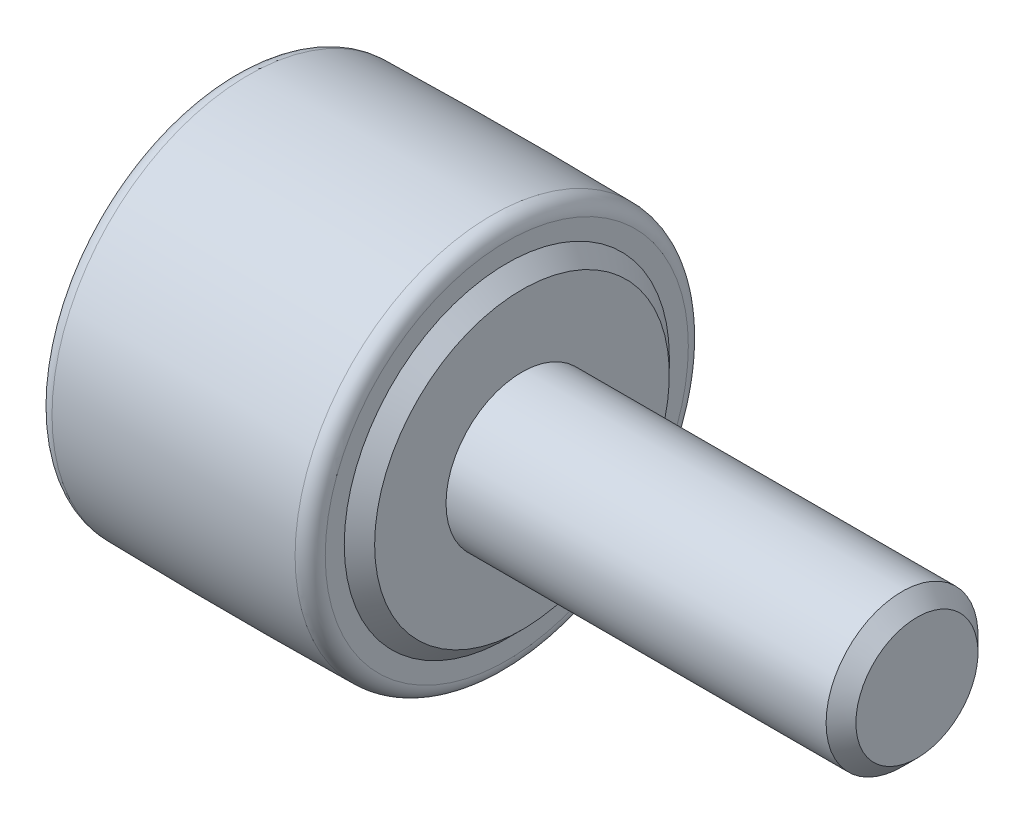
SolidWorks part; units mm, degrees
material "S45C"
ref_plane "Front Plane" through (0, 0, 0) normal (0, 0, 1) x (1, 0, 0)
ref_plane "Top Plane" through (0, 0, 0) normal (0, 1, 0) x (1, 0, 0)
ref_plane "Right Plane" through (0, 0, 0) normal (1, 0, 0) x (0, 0, -1)
ref_plane "Plane1" through (0, 0, 0) normal (0, 0, 1) x (1, 0, 0)
sketch "Sketch1" plane through (0, 0, 0) normal (0, 0, 1) x (1, 0, 0)
  line L0 (-10, 0) -> (-10, 4.85)
  line L1 (-10, 4.85) -> (-9.5, 5.35)
  line L2 (-9.5, 5.35) -> (-9.5, 5.9594)
  line L3 (-0.5, 5.9754) -> (-0.5, 5.35)
  line L4 (-0.5, 5.35) -> (0, 4.85)
  line L5 (0, 4.85) -> (0, 2.5)
  line L6 (0, 2.5) -> (12.5095, 2.5)
  line L7 (12.5095, 2.5) -> (13, 2.0095)
  line L8 (13, 2.0095) -> (13, 0)
  line L9 (13, 0) -> (-10, 0)
  line L10 (13, 0) -> (-10, 0) construction
  arc A0 (-9.5, 5.9594) -> (-9.009, 6.4593) centre (-9, 5.9594) cw
  arc A1 (-9.009, 6.4593) -> (-0.993, 6.4754) centre (-4.5, -243.5) cw
  arc A2 (-0.993, 6.4754) -> (-0.5, 5.9754) centre (-1, 5.9754) cw
revolve "Revolve1" add sketch "Sketch1" angle 360 about L10
ref_plane "Plane2" through (-10, 0, 0) normal (-1, 0, 0) x (0, 0, 1)
sketch "Sketch2" plane through (-10, 0, 0) normal (-1, 0, 0) x (0, 0, 1)
  line L0 (3.25, -0.5417) -> (3.25, 0.5417)
  line L1 (3.25, 0.5417) -> (-3.25, 0.5417)
  line L2 (-3.25, 0.5417) -> (-3.25, -0.5417)
  line L3 (-3.25, -0.5417) -> (3.25, -0.5417)
extrude "Cut-Extrude1" cut sketch "Sketch2" against normal blind 2
sketch "Sketch3" plane through (-0.5, 0, 0) normal (1, 0, 0) x (0, 0, -1)
  point P0 (0, 0)
